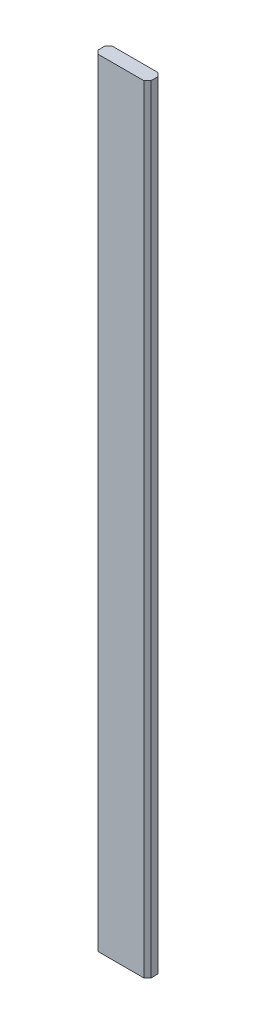
from build123d import *

# Parameters (mm, degrees)
SKETCH1_W           = 15
SKETCH1_H           = 220
BOSS_EXTRUDE1_DEPTH = 4
CHAMFER1_SIZE       = 1


with BuildPart() as part:
    # Sketch1 → Boss-Extrude1 (new body)
    with BuildSketch(Plane.XY):
        Rectangle(SKETCH1_W, SKETCH1_H)
    extrude(amount=BOSS_EXTRUDE1_DEPTH)

    # Chamfer1
    chamfer1_edges = [part.edges().sort_by_distance(p)[0] for p in [
        (7.5, 0, 4),
        (-7.5, 0, 4),
        (7.5, 0, 0),
        (-7.5, 0, 0),
    ]]
    chamfer(chamfer1_edges, length=CHAMFER1_SIZE)


solid = part.part
